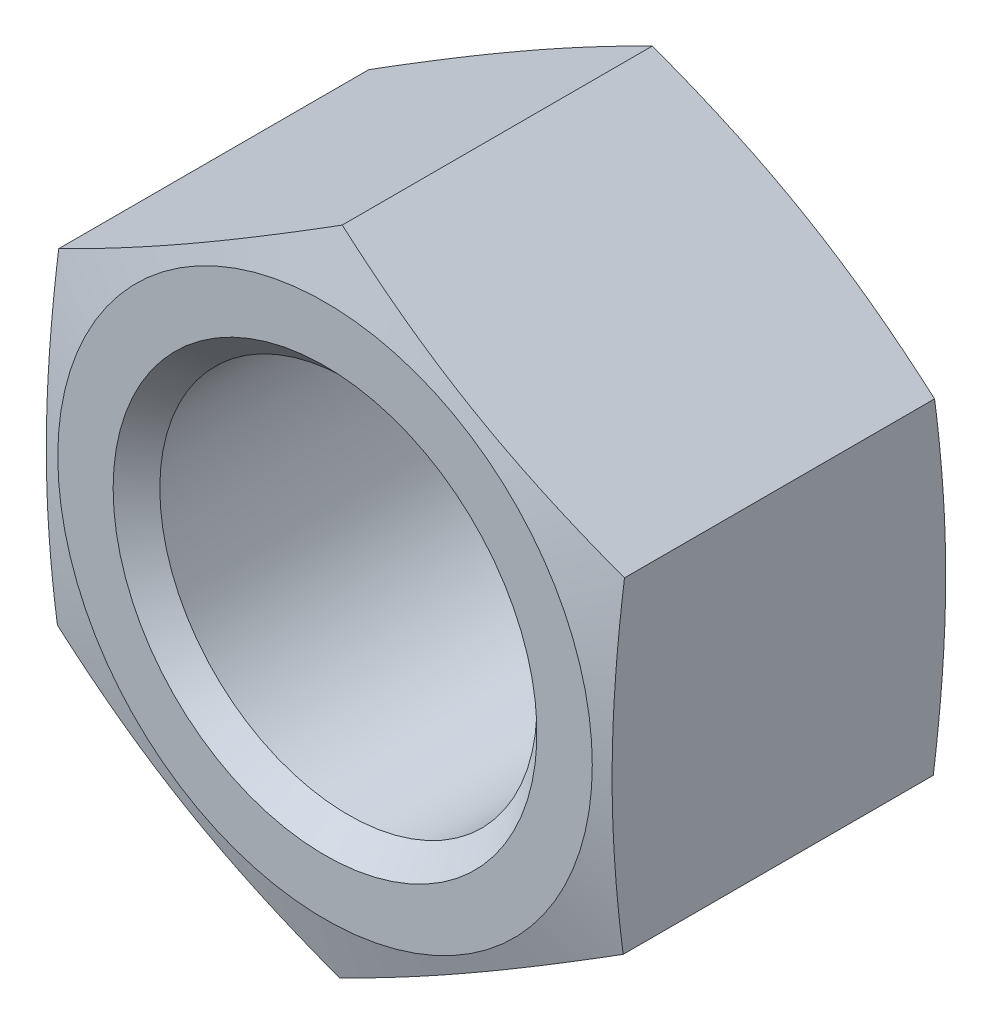
SolidWorks part; units mm, degrees
material "SAE2"
ref_plane "Plane1" through (0, 0, 0) normal (0, 0, 1) x (1, 0, 0)
ref_plane "Plane2" through (0, 0, 0) normal (0, 1, 0) x (1, 0, 0)
ref_plane "Plane3" through (0, 0, 0) normal (1, 0, 0) x (0, 0, -1)
sketch "Dimension Sketch" plane through (0, 0, 0) normal (0, 0, 1) x (1, 0, 0)
  line L0 (0, 0) -> (24.4249, 0)
  line L1 (24.4249, 0) -> (37.4249, 0)
  line L2 (37.4249, 0) -> (54.0249, 0)
  line L3 (-11.4286, 0) -> (0, 0)
  point P3 (12, 0)
  point P4 (1.5, 0)
  point P5 (20.03, 0)
  point P6 (10.8, 0)
  point P7 (6.4, 0)
  point P8 (18, 0)
  dimension "D1" = 11.4286
  dimension "D" = 12
  dimension "P" = 1.5
  dimension "e" = 20.03
  dimension "m" = 10.8
  dimension "mw" = 6.4
  dimension "s" = 18
  dimension "da" = 13
  dimension "dw" = 16.6
sketch "Sketch1" plane through (0, 0, 0) normal (0, 0, 1) x (1, 0, 0)
  line L0 (-26.8088, 0) -> (37.1748, 0) construction
  line L1 (0, 25.0215) -> (0, -25.0215) construction
  line L3 (0.0433, 10.9999) -> (-9.5046, 5.5374)
  line L4 (-9.5046, 5.5374) -> (-9.5478, -5.4625)
  line L5 (-9.5478, -5.4625) -> (-0.0433, -10.9999)
  line L6 (-0.0433, -10.9999) -> (9.5046, -5.5374)
  line L7 (9.5046, -5.5374) -> (9.5478, 5.4625)
  line L8 (9.5478, 5.4625) -> (0.0433, 10.9999)
  circle A0 centre (0, 0) radius 9.5263 construction
  circle A1 centre (0, 0) radius 6.35
  dimension "D" = 12.7
  dimension "e" = 22
extrude "Base-Extrude" add sketch "Sketch1" along normal blind 11.38
cosmetic thread "Cosmetic Thread1" parameters "D2"=12
sketch "Sketch2" plane through (0, 0, 0) normal (0, 0, -1) x (-1, 0, 0)
  circle A0 centre (0, 0) radius 9.5
  circle A1 centre (0, 0) radius 6.35 construction
  dimension "s" = 19
extrude "Cut-Extrude1" cut sketch "Sketch2" against normal through all draft 75 flip side to cut
sketch "Sketch3" plane through (0, 0, 11.38) normal (0, 0, 1) x (1, 0, 0)
  circle A0 centre (0, 0) radius 9
  dimension "D1" = 18
extrude "Cut-Extrude2" cut sketch "Sketch3" against normal through all draft 75 flip side to cut
chamfer "Chamfer1" distance 0.7857 angle 45 2 edges at (6.35, 0, 0) (6.35, 0, 11.38)
